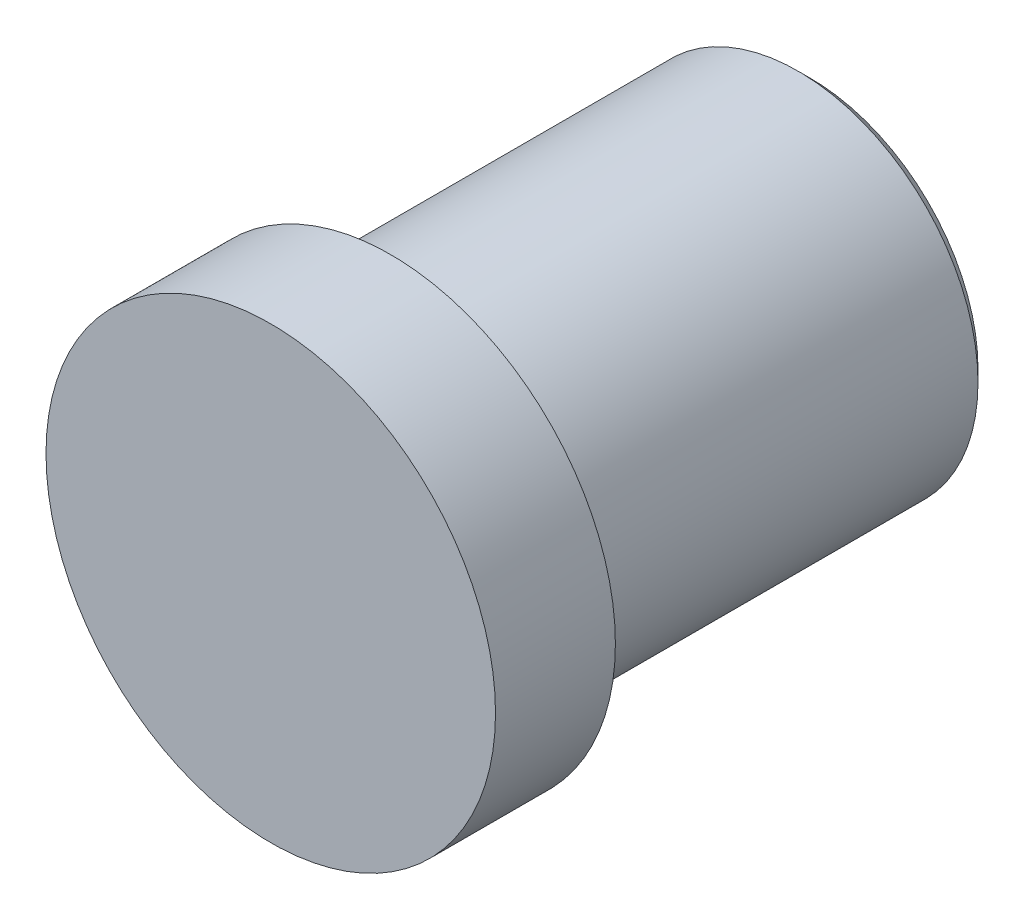
from build123d import *

# Parameters (mm, degrees)
SKETCH_1_R      = 30
EXTRUDE_1_DEPTH = 70
SKETCH_2_R      = 37.5
EXTRUDE_2_DEPTH = 20
CHAMFER_2_SIZE  = 2
SKETCH_3_W      = 1
SKETCH_3_H      = 2


with BuildPart() as part:
    # 草图1 → 凸台-拉伸1 (new body)
    with BuildSketch(Plane.XY):
        Circle(SKETCH_1_R)
    extrude(amount=EXTRUDE_1_DEPTH)

    # 草图2 → 凸台-拉伸2 (add)
    with BuildSketch(Plane.XY.offset(70)):
        Circle(SKETCH_2_R)
    extrude(amount=EXTRUDE_2_DEPTH)

    # 倒角2
    chamfer_2_edges = [part.edges().sort_by_distance(p)[0] for p in [
        (-30, 0, 0),
    ]]
    chamfer(chamfer_2_edges, length=CHAMFER_2_SIZE)

    # 草图3 → 切除-旋转1 (revolve, cut)
    with BuildSketch(Plane(origin=(0, 0, 0), x_dir=(1, 0, 0), z_dir=(0, 1, 0))):
        with Locations((29.5, -69)):
            Rectangle(SKETCH_3_W, SKETCH_3_H)
    revolve(axis=Axis((0, 0, 70), (0, 0, -1)), mode=Mode.SUBTRACT)


solid = part.part
